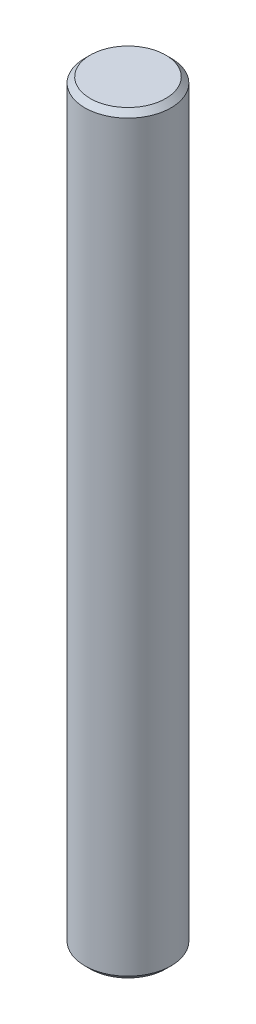
from build123d import *

# Parameters (mm, degrees)
SKETCH_1_R             = 4
EXTRUDE_1_DEPTH        = 70
CHAMFER_1_SIZE         = 0.5
HOLE_WIZARD_M4_1_D     = 3.3
HOLE_WIZARD_M4_1_DEPTH = 14.1
HOLE_WIZARD_M4_1_TIP   = 0.991420021


with BuildPart() as part:
    # 草图1 → 凸台-拉伸1 (new body)
    with BuildSketch(Plane(origin=(0, 0, 0), x_dir=(1, 0, 0), z_dir=(0, 1, 0))):
        with Locations(Location((0, 0, 0), (0, 0, 270))):
            Circle(SKETCH_1_R)
    extrude(amount=EXTRUDE_1_DEPTH)

    # 倒角1
    chamfer_1_edges = [part.edges().sort_by_distance(p)[0] for p in [
        (0, 0, -4),
        (0, 70, -4),
    ]]
    chamfer(chamfer_1_edges, length=CHAMFER_1_SIZE)

    # M4 螺纹孔1
    with Locations(Plane(origin=(0, 0, 0), x_dir=(-1, 0, 0), z_dir=(0, -1, 0))):
        with Locations((0, 0)):
            Hole(HOLE_WIZARD_M4_1_D / 2, depth=HOLE_WIZARD_M4_1_DEPTH)
            with Locations((0, 0, -(HOLE_WIZARD_M4_1_DEPTH + HOLE_WIZARD_M4_1_TIP / 2))):  # 118° drill point
                Cone(0, HOLE_WIZARD_M4_1_D / 2, HOLE_WIZARD_M4_1_TIP, mode=Mode.SUBTRACT)


solid = part.part
